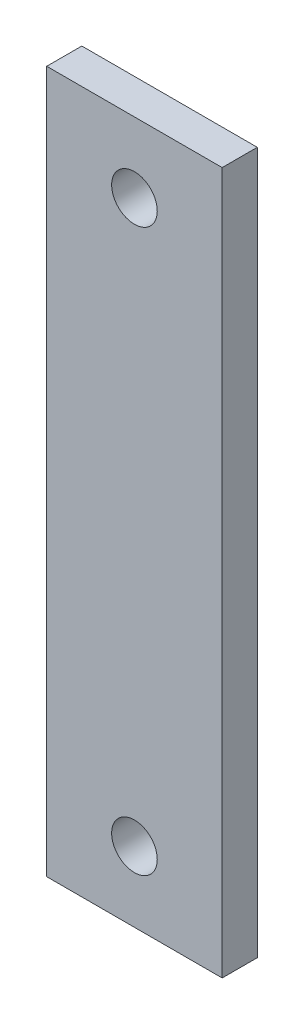
SolidWorks part; units mm, degrees
material "1023 碳钢板 (SS)"
ref_plane "前视基准面" through (0, 0, 0) normal (0, 0, 1) x (1, 0, 0)
ref_plane "上视基准面" through (0, 0, 0) normal (0, 1, 0) x (1, 0, 0)
ref_plane "右视基准面" through (0, 0, 0) normal (1, 0, 0) x (0, 0, -1)
sketch "草图1" plane through (0, 0, 0) normal (0, 0, 1) x (1, 0, 0)
  line L1 (-25, 100) -> (25, 100)
  line L2 (-25, 100) -> (-25, -100)
  line L3 (-25, -100) -> (25, -100)
  line L4 (25, 100) -> (25, -100)
  line L5 (-25, 100) -> (25, -100) construction
  line L6 (-25, -100) -> (25, 100) construction
  circle A0 centre (0, 80) radius 6.5
  circle A1 centre (0, -80) radius 6.5
  point P0 (0, 0)
  dimension "D5" = 13
  dimension "D1" = 50
  dimension "D2" = 200
  dimension "D3" = 160
  dimension "D4" = 20
extrude "凸台-拉伸1" add sketch "草图1" along normal blind 10
